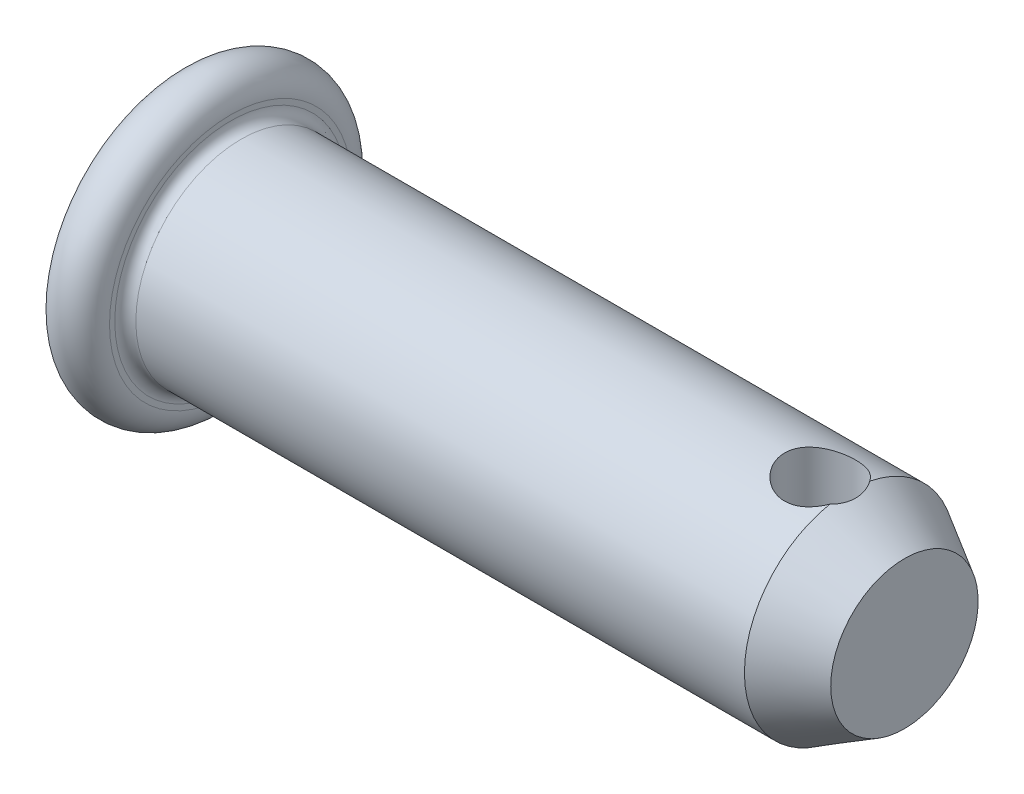
SolidWorks part; units mm, degrees
material "35钢"
ref_plane "前视" through (0, 0, 0) normal (0, 0, 1) x (1, 0, 0)
ref_plane "上视" through (0, 0, 0) normal (0, 1, 0) x (1, 0, 0)
ref_plane "右视" through (0, 0, 0) normal (1, 0, 0) x (0, 0, -1)
sketch "尺寸草图" plane through (0, 0, 0) normal (0, 0, 1) x (1, 0, 0)
  line L0 (0, 14) -> (0, 0)
  line L1 (0, 0) -> (32, 0)
  line L2 (32, 0) -> (36, 0) construction
  point P3 (0, 10)
  point P5 (2.5, 0)
  point P6 (0.5, 0)
  point P7 (30.5, 0)
  point P8 (4, 0)
  point P9 (0, 3.38)
sketch "草图1" plane through (0, 0, 0) normal (0, 0, 1) x (1, 0, 0)
  line L0 (0, 0) -> (10.7677, 0) construction
  line L1 (0, 0) -> (34.5, 0)
  line L2 (0, 0) -> (0, 5.75)
  line L4 (2.5, 5.75) -> (2.5, 5)
  line L5 (2.5, 5) -> (34.5, 5)
  line L6 (34.5, 5) -> (34.5, 0)
  arc A0 (0, 5.75) -> (2.5, 5.75) centre (1.25, 5.75) cw
revolve "基体-旋转" add sketch "草图1" angle 360 about L0
fillet "圆角1" radius 0.5 1 edges at (2.5, 0, 5)
chamfer "倒角1" distance 1.5 angle 60 1 edges at (34.5, 0, 5)
sketch "草图2" plane through (0, 0, 0) normal (0, 1, 0) x (1, 0, 0)
  line L0 (2.5, -5.5) -> (2.5, 5.5) construction
  circle A0 centre (30.5, 0) radius 1.69
extrude "切除-拉伸1" cut sketch "草图2" against normal mid plane 1000
equation "\"D4@草图1\" = \"K@尺寸草图\""
equation "\"D2@草图1\" = \"dk@尺寸草图\""
equation "\"D1@草图1\" = \"l@尺寸草图\""
equation "\"D3@草图1\" = \"d@尺寸草图\""
equation "\"D1@圆角1\" = \"r@尺寸草图\""
equation "\"D1@倒角1\" = \"c@尺寸草图\""
equation "\"D2@草图2\" = \"d1@尺寸草图\""
equation "\"lh@尺寸草图\" = \"l@尺寸草图\"-\"l-lh@尺寸草图\""
equation "\"D1@草图2\" = \"lh@尺寸草图\""
